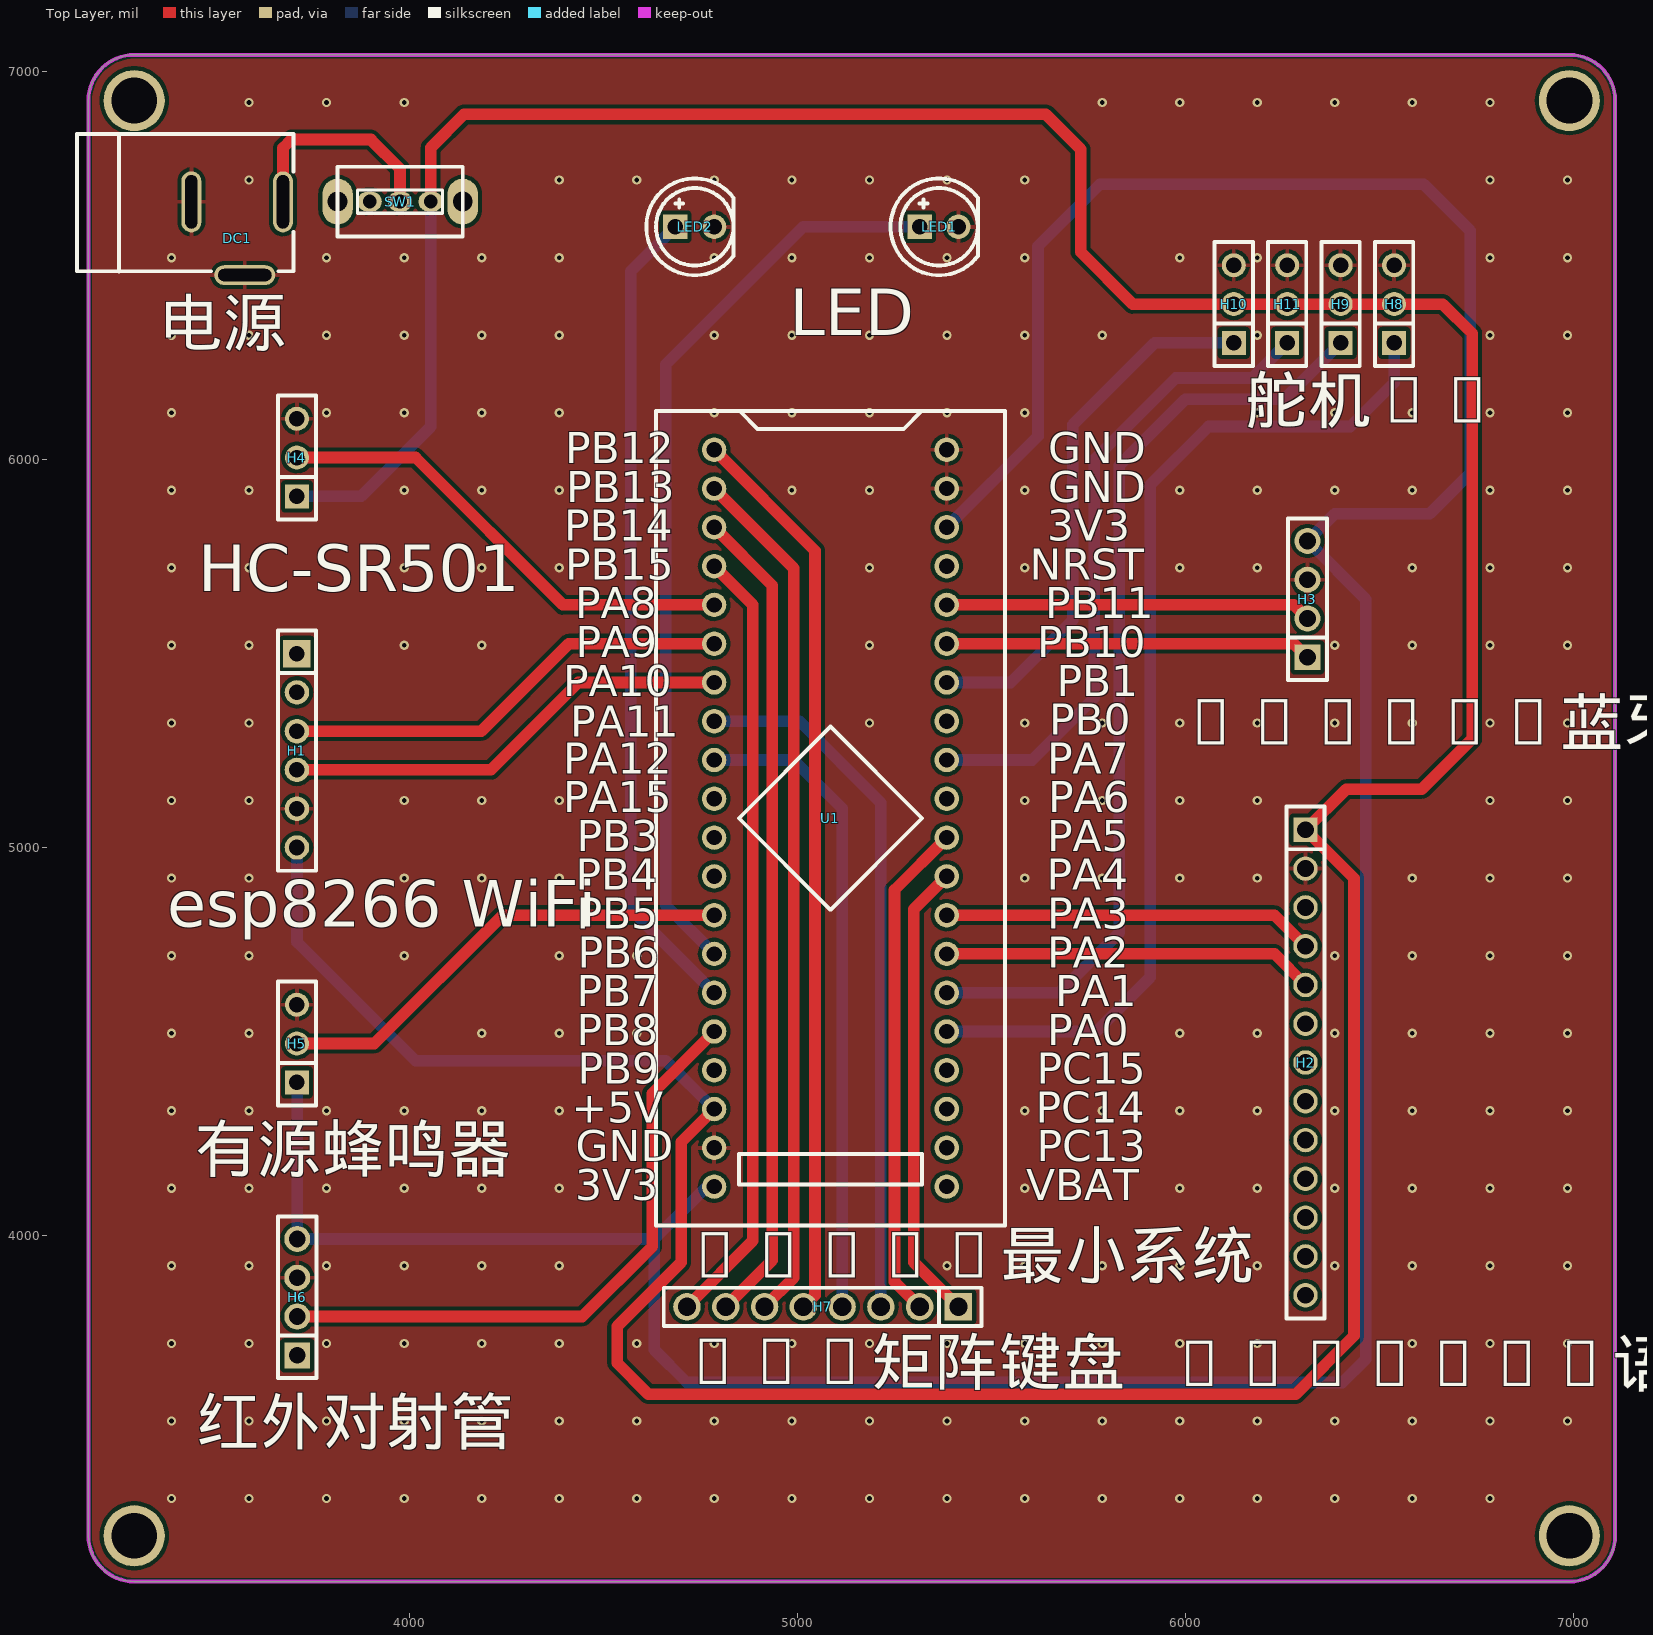
[diagram p0: Top Layer view]
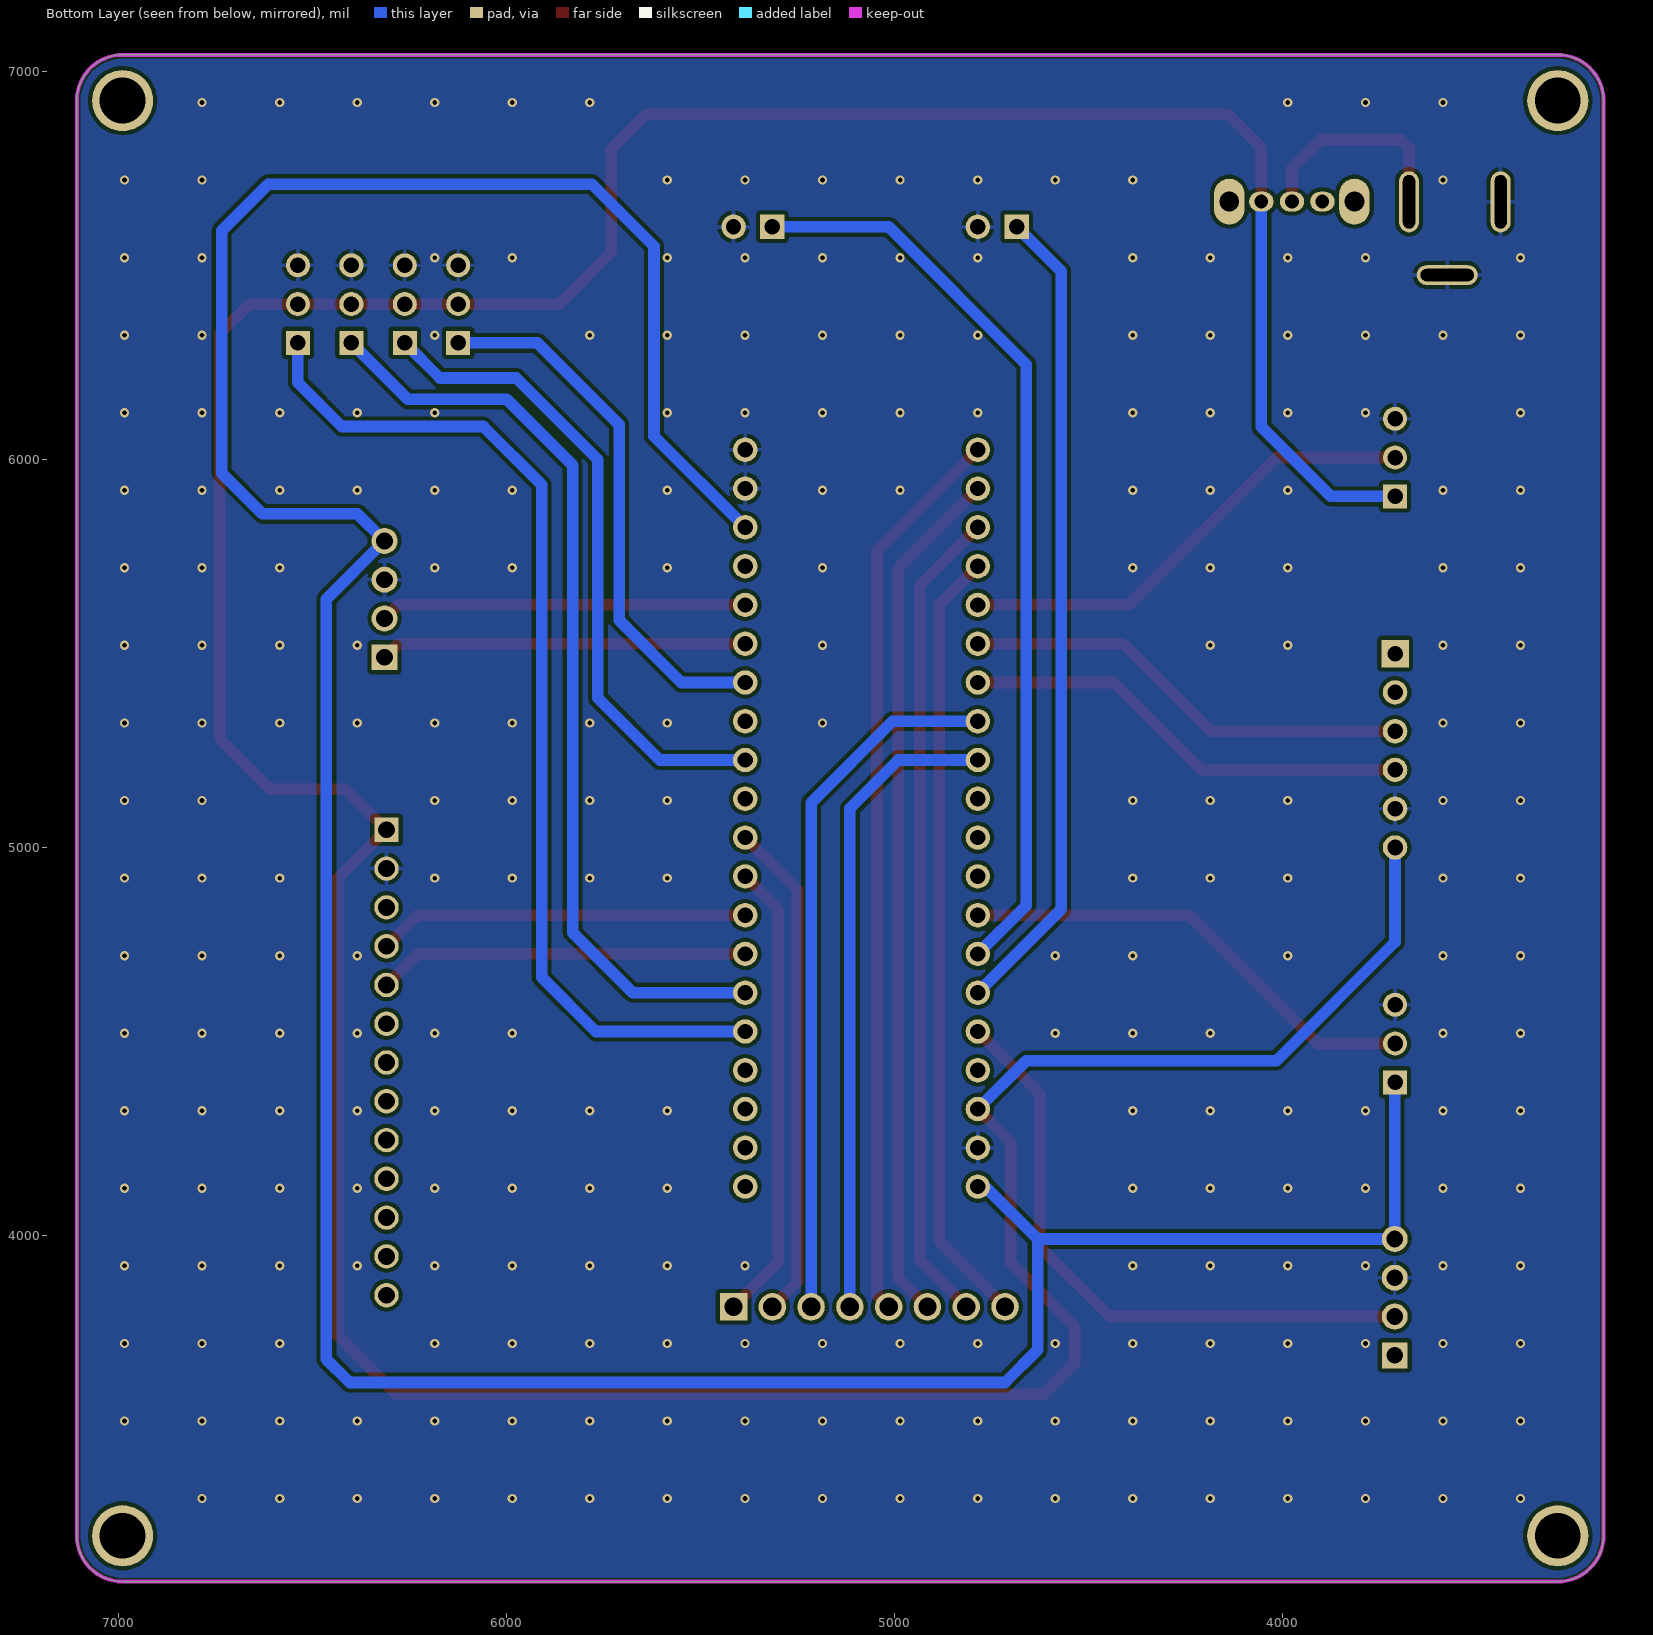
[diagram p1: Bottom Layer view, seen from below]
# Altium PCB MISC52050.pcbdoc
Units mil, origin at the board's own origin, x right, y up, seen from the top; angles counter-clockwise.
Board outline 3937.01 x 3937.01 mil, 2 copper layers (Top Layer, Bottom Layer), stack 62.206 mil thick; 16 components, 38 nets, 109 pads, 250 vias.

## Layer stack, top to bottom
Top Solder Mask Layer: solder mask 0.394, Dk 3.3
Top Layer: signal copper 1.379
Dielectric1: surface 59.449, FR4, Dk 4.5
Bottom Layer: signal copper 1.378
Bottom Solder Mask Layer: solder mask 0.394, Dk 3.3

## Board outline
6990.39,3106.5 ccw(c6990.39,3224.61) 7108.5,3224.61 7108.5,6925.39 ccw(c6990.39,6925.39) 6990.39,7043.5 3289.61,7043.5 ccw(c3289.61,6925.39) 3171.5,6925.39 3171.5,3224.61 ccw(c3289.61,3224.61) 3289.61,3106.5

## Design rules (kind name [scope] priority, off if disabled: settings)
BoardOutlineClearance copperThickness2oz_1 [All] p2 off: genericclearance=7.99 ignorepadtopadclearanceinfootprint=FALSE except(0: Arc-SplitContinuation Track-SplitContinuation SMDPad-SplitContinuation THPad-SplitContinuation Via-SplitContinuation Fill-SplitContinuation Region-SplitContinuation Poly-SplitContinuation Text-SplitContinuation Hole-SplitContinuation; 5.98: Arc-CutoutEdge Track-CutoutEdge SMDPad-CutoutEdge THPad-CutoutEdge Via-CutoutEdge Text-CutoutEdge; 6.89: Hole-OutlineEdge Hole-CutoutEdge; 10: Poly-OutlineEdge Poly-CutoutEdge; 11.81: Arc-OutlineEdge Track-OutlineEdge SMDPad-OutlineEdge THPad-OutlineEdge Via-OutlineEdge Fill-OutlineEdge Region-OutlineEdge Text-OutlineEdge Fill-CutoutEdge Region-CutoutEdge)
BoardOutlineClearance Plane_innerPlane_1 [All] p4 off: genericclearance=4.02 ignorepadtopadclearanceinfootprint=FALSE except(0: Arc-SplitContinuation Track-SplitContinuation SMDPad-SplitContinuation THPad-SplitContinuation Via-SplitContinuation Fill-SplitContinuation Region-SplitContinuation Poly-SplitContinuation Text-SplitContinuation Hole-SplitContinuation; 5.98: Arc-CutoutEdge Track-CutoutEdge SMDPad-CutoutEdge THPad-CutoutEdge Via-CutoutEdge Text-CutoutEdge; 6.89: Hole-OutlineEdge Hole-CutoutEdge; 10: Poly-OutlineEdge Poly-CutoutEdge; 11.81: Arc-OutlineEdge Track-OutlineEdge SMDPad-OutlineEdge THPad-OutlineEdge Via-OutlineEdge Fill-OutlineEdge Region-OutlineEdge Text-OutlineEdge Fill-CutoutEdge Region-CutoutEdge)
BoardOutlineClearance Copper_copperRegion_1 [All] p6 off: genericclearance=4.02 ignorepadtopadclearanceinfootprint=FALSE except(0: Arc-SplitContinuation Track-SplitContinuation SMDPad-SplitContinuation THPad-SplitContinuation Via-SplitContinuation Fill-SplitContinuation Region-SplitContinuation Poly-SplitContinuation Text-SplitContinuation Hole-SplitContinuation; 5.98: Arc-CutoutEdge Track-CutoutEdge SMDPad-CutoutEdge THPad-CutoutEdge Via-CutoutEdge Text-CutoutEdge; 6.89: Hole-OutlineEdge Hole-CutoutEdge; 10: Poly-OutlineEdge Poly-CutoutEdge; 11.81: Arc-OutlineEdge Track-OutlineEdge SMDPad-OutlineEdge THPad-OutlineEdge Via-OutlineEdge Fill-OutlineEdge Region-OutlineEdge Text-OutlineEdge Fill-CutoutEdge Region-CutoutEdge)
BoardOutlineClearance copperThickness1oz_1 [All] p8: genericclearance=4.02 ignorepadtopadclearanceinfootprint=FALSE except(0: Arc-SplitContinuation Track-SplitContinuation SMDPad-SplitContinuation THPad-SplitContinuation Via-SplitContinuation Fill-SplitContinuation Region-SplitContinuation Poly-SplitContinuation Text-SplitContinuation Hole-SplitContinuation; 5.98: Arc-CutoutEdge Track-CutoutEdge SMDPad-CutoutEdge THPad-CutoutEdge Via-CutoutEdge Text-CutoutEdge; 6.89: Hole-OutlineEdge Hole-CutoutEdge; 10: Poly-OutlineEdge Poly-CutoutEdge; 11.81: Arc-OutlineEdge Track-OutlineEdge SMDPad-OutlineEdge THPad-OutlineEdge Via-OutlineEdge Fill-OutlineEdge Region-OutlineEdge Text-OutlineEdge Fill-CutoutEdge Region-CutoutEdge)
Clearance copperThickness2oz [All] p1 off: gap=7.99 ignorepadtopadclearanceinfootprint=FALSE except(5.98: SMDPad-Track SMDPad-SMDPad THPad-Track SMDPad-THPad THPad-THPad Track-Via SMDPad-Via THPad-Via Via-Via Fill-SMDPad Region-SMDPad Fill-THPad Region-THPad Fill-Via Region-Via Fill-Fill Fill-Region Region-Region Arc-Track Arc-SMDPad Arc-THPad Arc-Via Fill-Arc Region-Arc Arc-Arc Text-Track SMDPad-Text Text-THPad Text-Via Fill-Text Region-Text Arc-Text Text-Text; 6.89: Hole-Track Hole-SMDPad Hole-THPad Hole-Via Fill-Hole Region-Hole Hole-Arc Hole-Text; 10: Poly-Track Poly-SMDPad Poly-THPad Poly-Via Poly-Fill Poly-Region Poly-Poly Poly-Arc Poly-Text Poly-Hole; 11.81: Fill-Track Region-Track)
Clearance Plane_innerPlane [All] p3 off: gap=4.02 ignorepadtopadclearanceinfootprint=FALSE except(5.98: SMDPad-Track SMDPad-SMDPad THPad-Track SMDPad-THPad THPad-THPad Track-Via SMDPad-Via THPad-Via Via-Via Fill-SMDPad Region-SMDPad Fill-THPad Region-THPad Fill-Via Region-Via Fill-Fill Fill-Region Region-Region Arc-Track Arc-SMDPad Arc-THPad Arc-Via Fill-Arc Region-Arc Arc-Arc Text-Track SMDPad-Text Text-THPad Text-Via Fill-Text Region-Text Arc-Text Text-Text; 6.89: Hole-Track Hole-SMDPad Hole-THPad Hole-Via Fill-Hole Region-Hole Hole-Arc Hole-Text; 10: Poly-Track Poly-SMDPad Poly-THPad Poly-Via Poly-Fill Poly-Region Poly-Poly Poly-Arc Poly-Text Poly-Hole; 11.81: Fill-Track Region-Track)
Clearance Copper_copperRegion [All] p5 off: gap=4.02 ignorepadtopadclearanceinfootprint=FALSE except(5.98: SMDPad-Track SMDPad-SMDPad THPad-Track SMDPad-THPad THPad-THPad Track-Via SMDPad-Via THPad-Via Via-Via Fill-SMDPad Region-SMDPad Fill-THPad Region-THPad Fill-Via Region-Via Fill-Fill Fill-Region Region-Region Arc-Track Arc-SMDPad Arc-THPad Arc-Via Fill-Arc Region-Arc Arc-Arc Text-Track SMDPad-Text Text-THPad Text-Via Fill-Text Region-Text Arc-Text Text-Text; 6.89: Hole-Track Hole-SMDPad Hole-THPad Hole-Via Fill-Hole Region-Hole Hole-Arc Hole-Text; 10: Poly-Track Poly-SMDPad Poly-THPad Poly-Via Poly-Fill Poly-Region Poly-Poly Poly-Arc Poly-Text Poly-Hole; 11.81: Fill-Track Region-Track)
Clearance copperThickness1oz [All] p7: gap=4.02 ignorepadtopadclearanceinfootprint=FALSE except(5.98: SMDPad-Track SMDPad-SMDPad THPad-Track SMDPad-THPad THPad-THPad Track-Via SMDPad-Via THPad-Via Via-Via Fill-SMDPad Region-SMDPad Fill-THPad Region-THPad Fill-Via Region-Via Fill-Fill Fill-Region Region-Region Arc-Track Arc-SMDPad Arc-THPad Arc-Via Fill-Arc Region-Arc Arc-Arc Text-Track SMDPad-Text Text-THPad Text-Via Fill-Text Region-Text Arc-Text Text-Text; 6.89: Hole-Track Hole-SMDPad Hole-THPad Hole-Via Fill-Hole Region-Hole Hole-Arc Hole-Text; 10: Poly-Track Poly-SMDPad Poly-THPad Poly-Via Poly-Fill Poly-Region Poly-Poly Poly-Arc Poly-Text Poly-Hole; 11.81: Fill-Track Region-Track)
DiffPairsRouting differentialPair [All] p1: maxlimit=6 minlimit=6 mostfreqgap=6 toplayer_minwidth=5 toplayer_prefwidth=10 toplayer_maxwidth=100 toplayer_mingap=6 toplayer_prefgap=6 toplayer_maxgap=6 bottomlayer_minwidth=5 bottomlayer_prefwidth=10 bottomlayer_maxwidth=100 bottomlayer_mingap=6 bottomlayer_prefgap=6 bottomlayer_maxgap=6 maxuncoupledlength=10
HoleToHoleClearance otherClearance [All] p1: gap=11.81 allowstackedmicrovias=TRUE
Length netLength [All] p1: minlimit=0 maxlimit=0
PasteMaskExpansion pasteMaskExpansion [All] p1: expansion=0
PlaneConnect innerPlane [All] p1: planeconnectstyle=Relief reliefexpansion=20 reliefentries=4 reliefconductorwidth=10 reliefairgap=10
PolygonConnect copperRegion [All] p1: connectstyle=Relief reliefconductorwidth=10 reliefentries=4 polygonreliefangle="90 Angle" airgapwidth=10 via.connectstyle=Relief via.reliefconductorwidth=10 via.reliefentries=4 via.polygonreliefangle="90 Angle" via.airgapwidth=10
RoutingVias viaSize [All] p1: holewidth=12.01 width=24.02 viastyle="Through Hole" minholewidth=11.81 minwidth=19.68 maxholewidth=248.03 maxwidth=393.7
SolderMaskExpansion solderMaskExpansion [IsVia] p1: expansion=-1000 istentingtop=TRUE
SolderMaskExpansion solderMaskExpansion [All] p2: expansion=2.01 istentingtop=FALSE
Width copperThickness2oz_2 [All] p1 off: maxlimit=100 minlimit=8 preferedwidth=10
Width copperThickness1oz_2 [All] p2: maxlimit=100 minlimit=5 preferedwidth=30

## Components (designator, comment, footprint, x,y, rotation, side; value= is the part's Value field where it differs from the comment)
DC1 "" DC-2.0 3550,6675 r180 top
H1 "" HDR-TH_6P-P2.54-V-F 3709.21,5249.48 r270 top
H2 "" HDR-TH_13P-P2.54-V-F 6310,4445 r270 top
H3 "" HDR-TH_4P-P2.54-V-F 6315,5640 r90 top
H4 "" HDR-TH_3P-P2.54-V-F 3709.21,6005 r90 top
H5 "" HDR-TH_3P-P2.54-V-F 3709.21,4493.95 r90 top
H6 "" HDR-TH_4P-P2.54-V-F 3710,3840 r90 top
H7 "" HDR-TH_8P-P2.54-V-F-1 5065,3815 r180 top
H8 "" HDR-TH_3P-P2.54-V-F 6538.48,6400.77 r90 top
H9 "" HDR-TH_3P-P2.54-V-F 6400.65,6400.77 r90 top
H10 "" HDR-TH_3P-P2.54-V-F 6125,6400.77 r90 top
H11 "" HDR-TH_3P-P2.54-V-F 6262.83,6400.77 r90 top
LED1 "" LED-TH_5mm 5365,6600 r0 top
LED2 "" LED-TH_5mm 4735,6600 r0 top
SW1 "" 拨动开关 3970,6665 r0 top
U1 "STM32F103C8T6-Card" CONN-TH_L53.3-W22.9_STM32F103C8T6-CARD 5085,5075 r270 top

## Footprints (in the part's own frame and the unit in brackets; to place one, negate y for a bottom-side part, rotate by r counter-clockwise, add the part's x,y. Pads: shape width x height; smd on the part's side, far side on the other; paste and mask are expansions set on the pad)
CONN-TH_L53.3-W22.9_STM32F103C8T6-CARD [mm]
  round 1.6 hole 1: 1(-24.13,-7.62) 2(-21.59,-7.62) 3(-19.05,-7.62) 4(-16.51,-7.62) 5(-13.97,-7.62) 6(-11.43,-7.62) 7(-8.89,-7.62) 8(-6.35,-7.62) 9(-3.81,-7.62) 10(-1.27,-7.62) 11(1.27,-7.62) 12(3.81,-7.62) 13(6.35,-7.62) 14(8.89,-7.62) 15(11.43,-7.62) 16(13.97,-7.62) 17(16.51,-7.62) 18(19.05,-7.62) 19(21.59,-7.62) 20(24.13,-7.62) 21(24.13,7.62) 22(21.59,7.62) 23(19.05,7.62) 24(16.51,7.62) 25(13.97,7.62) 26(11.43,7.62) 27(8.89,7.62) 28(6.35,7.62) 29(3.81,7.62) 30(1.27,7.62) 31(-1.27,7.62) 32(-3.81,7.62) 33(-6.35,7.62) 34(-8.89,7.62) 35(-11.43,7.62) 36(-13.97,7.62) 37(-16.51,7.62) 38(-19.05,7.62) 39(-21.59,7.62) 40(-24.13,7.62)
  silkscreen extent -26.67,-11.43 26.67,11.43
DC-2.0 [mil]
  oval 157.5x51.2 hole 31.5 slot 137.8 at 0 deg paste+0 mask+2: 2(-24.7,199.5)
  oval 51.2x157.5 hole 31.5 slot 137.8 at 90 deg paste+0 mask+2: 3(113.1,10.5) 4(-123.1,10.5)
  silkscreen extent -151,-165 408,190
HDR-TH_3P-P2.54-V-F [mil]
  rect 62x62 hole 40.16: 1(-100,0)
  round 62 hole 40.16: 2(0,0) 3(100,0)
  silkscreen extent -160,-49 160,49
HDR-TH_4P-P2.54-V-F [mm]
  rect 1.7x1.7 hole 1.1: 1(-3.81,0)
  round 1.7 hole 1.1: 2(-1.27,0) 3(1.27,0) 4(3.81,0)
  silkscreen extent -5.29,-1.27 5.29,1.27
HDR-TH_6P-P2.54-V-F [mm]
  rect 1.8x1.8 hole 1.02: 1(-6.35,0)
  round 1.6 hole 1.02: 2(-3.81,0) 3(-1.27,0) 4(1.27,0) 5(3.81,0) 6(6.35,0)
  silkscreen extent -7.87,-1.25 7.87,1.25
HDR-TH_8P-P2.54-V-F-1 [mm]
  rect 1.8x1.8 hole 1.2: 1(-8.89,0)
  round 1.8 hole 1.2: 2(-6.35,0) 3(-3.81,0) 4(-1.27,0) 5(1.27,0) 6(3.81,0) 7(6.35,0) 8(8.89,0)
  silkscreen extent -10.41,-1.25 10.41,1.25
HDR-TH_13P-P2.54-V-F [mm]
  rect 1.6x1.6 hole 1.1: 1(-15.24,0)
  round 1.6 hole 1.1: 2(-12.7,0) 3(-10.16,0) 4(-7.62,0) 5(-5.08,0) 6(-2.54,0) 7(0,0) 8(2.54,0) 9(5.08,0) 10(7.62,0) 11(10.16,0) 12(12.7,0) 13(15.24,0)
  silkscreen extent -16.76,-1.25 16.76,1.25
LED-TH_5mm [mm]
  rect 1.6x1.6 hole 1 paste+0 mask+0.051: 1(-1.27,0)
  round 1.6 hole 1 paste+0 mask+0.051: 2(1.27,0)
  silkscreen extent -3.17,-3.17 2.54,3.17
拨动开关 [mil]
  oval 63x51.2 hole 35.4 paste+0 mask+2: 1(-73.4,0) 2(5,0) 3(84,0)
  oval 78.7x118.1 hole 51.2 paste+0 mask+2: 4(166.7,0) 5(-156.1,0)
  silkscreen extent -156,-90 167,90

## Free pads (board coordinates)
  round 157.48 hole 118.11: 1(3289.61,6925.39) 1(3289.61,3224.61) 1(6990.39,6925.39) 1(6990.39,3224.61)

## Via types
v1: diameter 24.02, hole 12, Top Layer to Bottom Layer, 250 vias

## Nets (pads, with @x,y where several pads share a name; then routed paths per layer and width w, separated by ;. In a path a pad name is that pad's centre, name@x,y a point inside that pad or via, vN(x,y) a via of type N, cw(c..) or ccw(c..) an arc to the next point about the centre after c; other vN are vias at no path point)
$1N18271: DC1.4 SW1.2 | length 565.6
  Top Layer w30: DC1.4 3673.1,6803.1 3695,6825 3900,6825 3975,6750 SW1.2
+5V: H1.6 H2.1 H4.1 H8.2 H9.2 H10.2 H11.2 SW1.3 U1.18 | length 11430.7
  Top Layer w30: SW1.3 4054,6804 4140,6890 5640,6890 5730,6800 5730,6535 5864.23,6400.77 H10.2 H11.2 H9.2 H8.2 6664.23,6400.77 6740,6325 6740,5280 6610,5150 6415,5150 H2.1 6435,4920 6435,3740 6285,3590 4615,3590 4535,3670 4535,3765 4700,3930 4700,4240 U1.18
  Bottom Layer w30: H1.6 3709.21,4755.79 4015,4450 4660,4450 U1.18 ; H4.1 3875,5905 4054,6084 SW1.3
GND: DC1.2 DC1.3 H1.5 H2.2 H3.3 H4.3 H5.3 H6.3 H8.3 H9.3 H10.3 H11.3 LED1.2 LED2.2 U1.19 U1.39 U1.40
  other v1: 3385.6,3320.6 3585.6,3320.6 3785.6,3320.6 3985.6,3320.6 4185.6,3320.6 4385.6,3320.6 4585.6,3320.6 4785.6,3320.6 4985.6,3320.6 5185.6,3320.6 5385.6,3320.6 5585.6,3320.6 5785.6,3320.6 5985.6,3320.6 6185.6,3320.6 6385.6,3320.6 6585.6,3320.6 6785.6,3320.6 3385.6,3520.6 3585.6,3520.6 3785.6,3520.6 3985.6,3520.6 4185.6,3520.6 4385.6,3520.6 4585.6,3520.6 4785.6,3520.6 4985.6,3520.6 5185.6,3520.6 5385.6,3520.6 5585.6,3520.6 5785.6,3520.6 5985.6,3520.6 6185.6,3520.6 6385.6,3520.6 6585.6,3520.6 6785.6,3520.6 6985.6,3520.6 3385.6,3720.6 3585.6,3720.6 3785.6,3720.6 3985.6,3720.6 4185.6,3720.6 4385.6,3720.6 4585.6,3720.6 4785.6,3720.6 4985.6,3720.6 5185.6,3720.6 5385.6,3720.6 5585.6,3720.6 5785.6,3720.6 5985.6,3720.6 6185.6,3720.6 6585.6,3720.6 6785.6,3720.6 6985.6,3720.6 3385.6,3920.6 3585.6,3920.6 3785.6,3920.6 3985.6,3920.6 4185.6,3920.6 4385.6,3920.6 5385.6,3920.6 5585.6,3920.6 5785.6,3920.6 5985.6,3920.6 6185.6,3920.6 6385.6,3920.6 6585.6,3920.6 6785.6,3920.6 6985.6,3920.6 3385.6,4120.6 3585.6,4120.6 3785.6,4120.6 3985.6,4120.6 4185.6,4120.6 4385.6,4120.6 5585.6,4120.6 5785.6,4120.6 5985.6,4120.6 6185.6,4120.6 6385.6,4120.6 6585.6,4120.6 6785.6,4120.6 6985.6,4120.6 3385.6,4320.6 3585.6,4320.6 3785.6,4320.6 3985.6,4320.6 4185.6,4320.6 4385.6,4320.6 5585.6,4320.6 5785.6,4320.6 5985.6,4320.6 6185.6,4320.6 6385.6,4320.6 6585.6,4320.6 6785.6,4320.6 6985.6,4320.6 3385.6,4520.6 3585.6,4520.6 4185.6,4520.6 4385.6,4520.6 4585.6,4520.6 5985.6,4520.6 6185.6,4520.6 6385.6,4520.6 6585.6,4520.6 6785.6,4520.6 6985.6,4520.6 3385.6,4720.6 3585.6,4720.6 3985.6,4720.6 4385.6,4720.6 4585.6,4720.6 6385.6,4720.6 6585.6,4720.6 6785.6,4720.6 6985.6,4720.6 3385.6,4920.6 3585.6,4920.6 3985.6,4920.6 4185.6,4920.6 4385.6,4920.6 5585.6,4920.6 5785.6,4920.6 5985.6,4920.6 6185.6,4920.6 6585.6,4920.6 6785.6,4920.6 6985.6,4920.6 3385.6,5120.6 3585.6,5120.6 3985.6,5120.6 4185.6,5120.6 4385.6,5120.6 5585.6,5120.6 5785.6,5120.6 5985.6,5120.6 6185.6,5120.6 6785.6,5120.6 6985.6,5120.6 3385.6,5320.6 3585.6,5320.6 5185.6,5320.6 5585.6,5320.6 5785.6,5320.6 5985.6,5320.6 6185.6,5320.6 6385.6,5320.6 6585.6,5320.6 6785.6,5320.6 6985.6,5320.6 3385.6,5520.6 3585.6,5520.6 3985.6,5520.6 4185.6,5520.6 5185.6,5520.6 6385.6,5520.6 6585.6,5520.6 6785.6,5520.6 6985.6,5520.6 3385.6,5720.6 3585.6,5720.6 3985.6,5720.6 4185.6,5720.6 4385.6,5720.6 5185.6,5720.6 5585.6,5720.6 5985.6,5720.6 6185.6,5720.6 6585.6,5720.6 6785.6,5720.6 6985.6,5720.6 3385.6,5920.6 3585.6,5920.6 3985.6,5920.6 4185.6,5920.6 4385.6,5920.6 4985.6,5920.6 5185.6,5920.6 5585.6,5920.6 5985.6,5920.6 6185.6,5920.6 6385.6,5920.6 6585.6,5920.6 6785.6,5920.6 6985.6,5920.6 3385.6,6120.6 3785.6,6120.6 3985.6,6120.6 4185.6,6120.6 4385.6,6120.6 4785.6,6120.6 4985.6,6120.6 5185.6,6120.6 5385.6,6120.6 5585.6,6120.6 6185.6,6120.6 6385.6,6120.6 6585.6,6120.6 6785.6,6120.6 6985.6,6120.6 3385.6,6320.6 3585.6,6320.6 3785.6,6320.6 3985.6,6320.6 4185.6,6320.6 4385.6,6320.6 4785.6,6320.6 4985.6,6320.6 5185.6,6320.6 5385.6,6320.6 5585.6,6320.6 5785.6,6320.6 6185.6,6320.6 6785.6,6320.6 6985.6,6320.6 3385.6,6520.6 3785.6,6520.6 3985.6,6520.6 4185.6,6520.6 4385.6,6520.6 4785.6,6520.6 4985.6,6520.6 5185.6,6520.6 5385.6,6520.6 5585.6,6520.6 5985.6,6520.6 6185.6,6520.6 6785.6,6520.6 6985.6,6520.6 3585.6,6720.6 4385.6,6720.6 4585.6,6720.6 4785.6,6720.6 4985.6,6720.6 5185.6,6720.6 5385.6,6720.6 5585.6,6720.6 6785.6,6720.6 6985.6,6720.6 3585.6,6920.6 3785.6,6920.6 3985.6,6920.6 5785.6,6920.6 5985.6,6920.6 6185.6,6920.6 6385.6,6920.6 6585.6,6920.6 6785.6,6920.6
NRST: U1.37
PA0: H8.1 U1.25 | length 2692.9
  Bottom Layer w30: U1.25 5770,4525 5910,4665 5910,5935 6060,6085 6425,6085 6538.48,6198.48 H8.1
PA1: H9.1 U1.26 | length 2415.7
  Bottom Layer w30: U1.26 5675,4625 5830,4780 5830,5985 6000,6155 6254.88,6155 H9.1
PA2: H2.5 U1.27 | length 958.1
  Top Layer w30: U1.27 6230,4725 H2.5
PA3: H2.4 U1.28 | length 958.1
  Top Layer w30: U1.28 6230,4825 H2.4
PA4: H7.1 U1.29 | length 1192.8
  Top Layer w30: U1.29 5300,4840 5300,3930 H7.1
PA5: H7.2 U1.30 | length 1292.8
  Top Layer w30: H7.2 5250,3880 5250,4890 U1.30
PA6: U1.31
PA7: H11.1 U1.32 | length 1683.7
  Bottom Layer w30: U1.32 5605,5225 5765,5385 5765,6000 5975,6210 6172.06,6210 H11.1
PA8: H4.2 U1.5 | length 1233.2
  Top Layer w30: H4.2 4015,6005 4395,5625 U1.5
PA9: H1.3 U1.6 | length 1169.2
  Top Layer w30: H1.3 4184.48,5299.48 4410,5525 U1.6
PA10: H1.4 U1.7 | length 1169.2
  Top Layer w30: H1.4 4209.48,5199.48 4435,5425 U1.7
PA11: H7.3 U1.8 | length 1817
  Bottom Layer w30: U1.8 5005,5325 5215,5115 H7.3
PA12: H7.4 U1.9 | length 1666.8
  Bottom Layer w30: U1.9 4990,5225 5115,5100 H7.4
PA15: U1.10
PB0: U1.33
PB1: H10.1 U1.34 | length 1398.6
  Bottom Layer w30: U1.34 5550,5425 5710,5585 5710,6090 5920.77,6300.77 H10.1
PB3: U1.11
PB4: U1.12
PB5: H5.2 U1.13 | length 1212.9
  Top Layer w30: H5.2 3908.95,4493.95 4240,4825 U1.13
PB6: LED1.1 U1.14 | length 2373.8
  Bottom Layer w30: U1.14 4660,4850 4660,6245 5015,6600 LED1.1
PB7: LED2.1 U1.15 | length 2111.7
  Bottom Layer w30: LED2.1 4570,6485 4570,4840 U1.15
PB8: H6.2 U1.16 | length 1610.8
  Top Layer w30: H6.2 4445,3790 4625,3970 4625,4365 U1.16
PB9: U1.17
PB10: H3.1 U1.35 | length 944.5
  Top Layer w30: U1.35 6280,5525 H3.1
PB11: H3.2 U1.36 | length 944.5
  Top Layer w30: U1.36 6280,5625 H3.2
PB12: H7.5 U1.1 | length 2330.1
  Top Layer w30: U1.1 5045,5765 5045,3845 H7.5
PB13: H7.6 U1.2 | length 2226
  Top Layer w30: U1.2 4990,5720 4990,3890 H7.6
PB14: H7.7 U1.3 | length 2121.8
  Top Layer w30: U1.3 4935,5675 4935,3935 H7.7
PB15: H7.8 U1.4 | length 2021.8
  Top Layer w30: H7.8 4885,3985 4885,5625 U1.4
PC13: U1.22
PC14: U1.23
PC15: U1.24
VBAT: U1.21
VCC: H3.4 H5.1 H6.4 U1.20 U1.38 | length 9057.9
  Bottom Layer w30: H5.1 3710,4393.16 H6.4 4630.83,3990 ; U1.20 4765.83,4125 4630.83,3990 ; U1.38 5620,6060 5620,6550 5780,6710 6615,6710 6735,6590 6735,5965 6630,5860 6385,5860 H3.4 6465,5640 6465,3680 6405,3620 4715,3620 4630.83,3704.17 4630.83,3990
pads on no net: H1.1 H1.2 H2.3 H2.6 H2.7 H2.8 H2.9 H2.10 H2.11 H2.12 H2.13 H6.1 SW1.1 SW1.4 SW1.5

## Polygon pours and split planes (outlines as drawn)
GND on Bottom Layer (solid, remove dead copper, pour order 2): 3100,7165 3100,3000 7275,3000 7275,7165
GND on Top Layer (solid, remove dead copper, pour order 0): 3000,7145 3000,3075 7385,3075 7385,7145

## Keep-outs
Board Outline Layer:
  the board outline again, w10

## Silkscreen, mask and mechanical layers (free items; w line width, h text height)
Top Silkscreen Layer:
  text "LED" at 4980,6320 h120
  text "电源" at 3355,6295 h120
  text "舵机*4" at 6155,6095 h120
  text "PB12" at 4400.64,5990 h80
  text "GND" at 5646.65,5990 h80
  text "PB13" at 4403.85,5890 h80
  text "GND" at 5646.65,5890 h80
  text "PB14" at 4398.34,5790 h80
  text "3V3" at 5644.45,5790 h80
  text "PB15" at 4400.64,5690 h80
  text "NRST" at 5598.65,5690 h80
  text "HC-SR501" at 3455,5660 h120
  text "PA8" at 4426.24,5590 h80
  text "PB11" at 5639.05,5590 h80
  text "PA9" at 4428.44,5490 h80
  text "PB10" at 5618.85,5490 h80
  text "PA10" at 4396.14,5390 h80
  text "PB1" at 5669.15,5390 h80
  text "PB0" at 5648.95,5290 h80
  text "PA11" at 4414.55,5285 h80
  text "JDY-31蓝牙模块" at 5985,5265 h120
  text "PA12" at 4396.14,5190 h80
  text "PA7" at 5644.45,5190 h80
  text "PA15" at 4396.14,5090 h80
  text "PA6" at 5646.65,5090 h80
  text "PB3" at 4430.74,4990 h80
  text "PA5" at 5644.45,4990 h80
  text "PB4" at 4428.44,4890 h80
  text "PA4" at 5642.15,4890 h80
  text "esp8266 WiFi" at 3375,4795 h120
  text "PB5" at 4430.74,4790 h80
  text "PA3" at 5644.45,4790 h80
  text "PB6" at 4432.94,4690 h80
  text "PA2" at 5644.45,4690 h80
  text "PB7" at 4430.74,4590 h80
  text "PA1" at 5664.65,4590 h80
  text "PB8" at 4430.74,4490 h80
  text "PA0" at 5644.45,4490 h80
  text "PB9" at 4432.94,4390 h80
  text "PC15" at 5616.55,4390 h80
  text "+5V" at 4417.24,4290 h80
  text "PC14" at 5614.25,4290 h80
  text "GND" at 4428.44,4190 h80
  text "PC13" at 5616.55,4190 h80
  text "有源蜂鸣器" at 3445,4165 h120
  text "3V3" at 4426.24,4090 h80
  text "VBAT" at 5589.65,4090 h80
  text "STM32最小系统" at 4705,3890 h120
  text "4X4矩阵键盘" at 4700,3615 h120
  text "SNR8016语音模块" at 5955,3610 h120
  text "红外对射管" at 3450,3460 h120